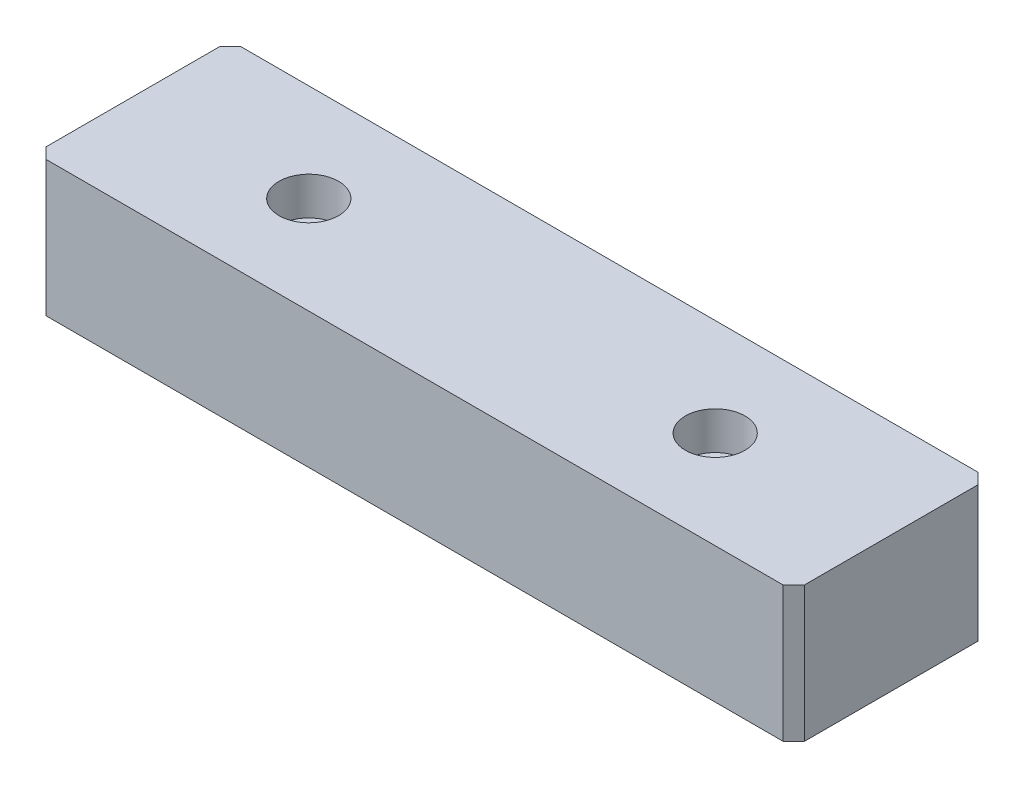
from build123d import *

# Parameters (mm, degrees)
SKETCH_1_W                = 140
SKETCH_1_H                = 36
EXTRUDE_1_DEPTH           = 25
HOLE_WIZARD_1_D           = 6.6
HOLE_WIZARD_1_CBORE_D     = 11
HOLE_WIZARD_1_CBORE_DEPTH = 7
CHAMFER_1_SIZE            = 2


with BuildPart() as part:
    # 草图1 → 凸台-拉伸1 (new body)
    with BuildSketch(Plane(origin=(0, 0, 0), x_dir=(1, 0, 0), z_dir=(0, 1, 0))):
        with Locations((70, 18)):
            Rectangle(SKETCH_1_W, SKETCH_1_H)
    extrude(amount=EXTRUDE_1_DEPTH)

    # 打孔尺寸(%根据)内六角圆柱头螺钉的类型1 (through all)
    with Locations(Plane(origin=(0, 25, 0), x_dir=(1, 0, 0), z_dir=(0, 1, 0))):
        with Locations((32.5, 18), (107.5, 18)):
            CounterBoreHole(HOLE_WIZARD_1_D / 2, HOLE_WIZARD_1_CBORE_D / 2, HOLE_WIZARD_1_CBORE_DEPTH)

    # 倒角1
    chamfer_1_edges = [part.edges().sort_by_distance(p)[0] for p in [
        (0, 12.5, -36),
        (140, 12.5, -36),
        (140, 12.5, 0),
        (0, 12.5, 0),
    ]]
    chamfer(chamfer_1_edges, length=CHAMFER_1_SIZE)


solid = part.part
